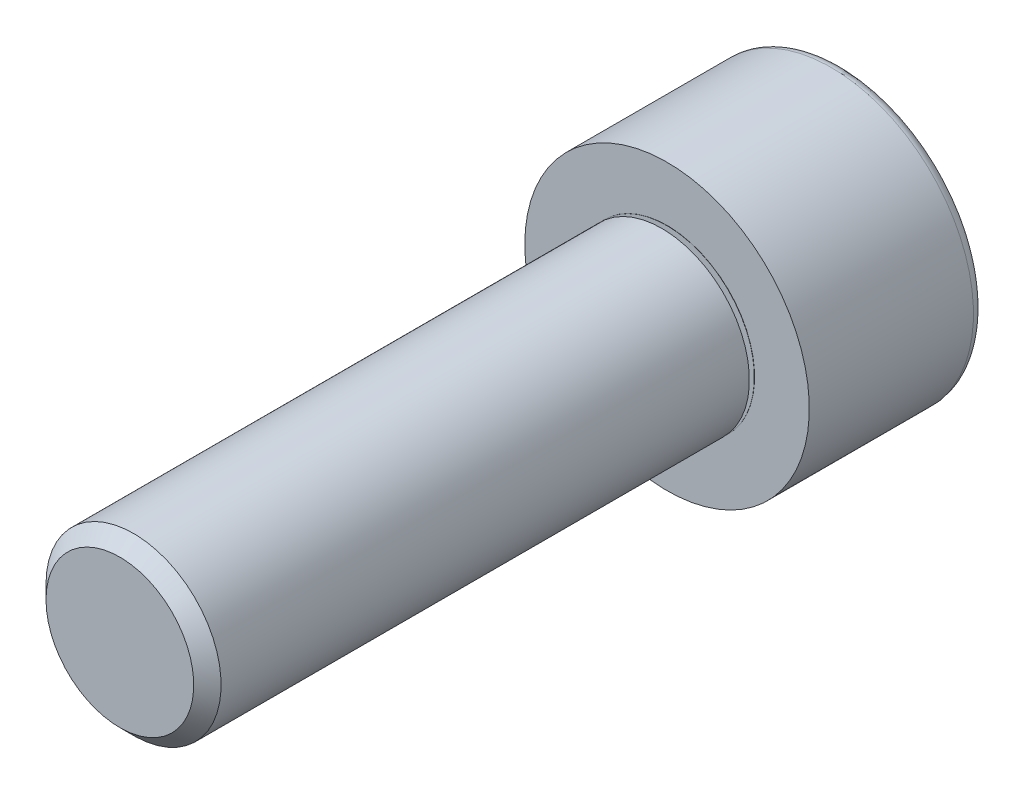
from build123d import *

# Parameters (mm, degrees)
CUT_EXTRUDE1_DEPTH = 3


with BuildPart() as part:
    # Logo3_bib1 → Revolve1 (revolve)
    with BuildSketch(Plane(origin=(0, 0, 0), x_dir=(-1, 0, 0), z_dir=(0, -1, 0))):
        with BuildLine():
            Line((0, -25), (0, 8))
            Line((0, 8), (6, 8))
            ThreePointArc((6, 8), (6.353553391, 7.853553391), (6.5, 7.5))
            Line((6.5, 7.5), (6.5, 0))
            Line((6.5, 0), (4, 0))
            Line((4, 0), (4, -0.01))
            Line((4, -0.01), (3.488425636, -0.01))
            ThreePointArc((3.488425636, -0.01), (3.468729481, -0.026527036), (3.481585234, -0.048793852))
            Line((3.481585234, -0.048793852), (4, -0.237481396))
            Line((4, -0.237481396), (4, -24.375))
            Line((4, -24.375), (3.375, -25))
            Line((3.375, -25), (0, -25))
        make_face()
    revolve(axis=Axis((0, 0, -10.585154653), (0, 0, 1)))

    # Logo3_bib2 → Cut-Extrude1 (cut)
    with BuildSketch(Plane(origin=(0, 0, -8), x_dir=(1, 0, 0), z_dir=(0, 0, -1))):
        Polygon((3.464101615, 0), (1.732050808, 3), (-1.732050808, 3), (-3.464101615, 0), (-1.732050808, -3), (1.732050808, -3), align=None)
    extrude(amount=-CUT_EXTRUDE1_DEPTH, mode=Mode.SUBTRACT)


solid = part.part
